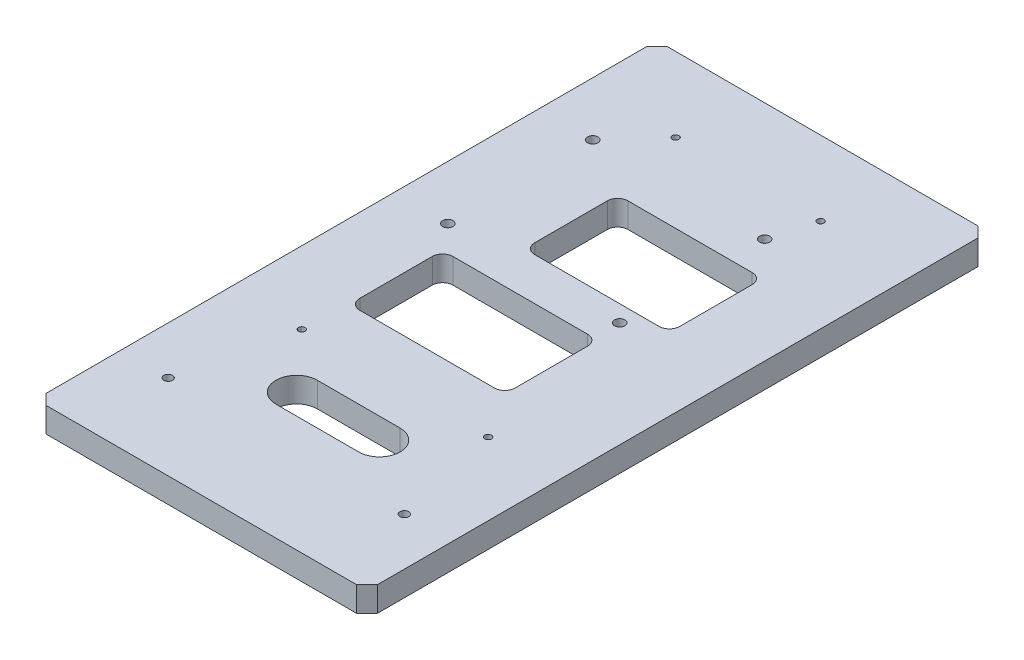
SolidWorks part; units mm, degrees
ref_plane "前视基准面" through (0, 0, 0) normal (0, 0, 1) x (1, 0, 0)
ref_plane "上视基准面" through (0, 0, 0) normal (0, 1, 0) x (1, 0, 0)
ref_plane "右视基准面" through (0, 0, 0) normal (1, 0, 0) x (0, 0, -1)
sketch "草图1" plane through (0, 0, 0) normal (0, 1, 0) x (1, 0, 0)
  line L1 (-80, 150) -> (80, 150)
  line L2 (-80, 150) -> (-80, -150)
  line L3 (-80, -150) -> (80, -150)
  line L4 (80, 150) -> (80, -150)
  line L5 (-80, 150) -> (80, -150) construction
  line L6 (-80, -150) -> (80, 150) construction
  point P0 (0, 0)
  dimension "D1" = 160
  dimension "D2" = 300
extrude "凸台-拉伸1" add sketch "草图1" along normal blind 12
sketch "草图6" plane through (0, 12, 0) normal (0, 1, 0) x (1, 0, 0)
  line L0 (-20, -84) -> (20, -84) construction
  line L1 (-20, -74) -> (20, -74)
  line L2 (-20, -94) -> (20, -94)
  line L3 (-80, 150) -> (-80, -150) construction
  line L5 (80, 150) -> (-80, 150) construction
  arc A0 (-20, -74) -> (-20, -94) centre (-20, -84) ccw
  arc A1 (20, -94) -> (20, -74) centre (20, -84) ccw
  point P2 (0, -84)
  dimension "D1" = 234
  dimension "D2" = 20
  dimension "D3" = 40
  dimension "D4" = 80
extrude "切除-拉伸1" cut sketch "草图6" against normal through all
hole_wizard "打孔尺寸(%根据)开槽圆柱头螺钉的类型3" positions "草图12" profile "草图11" counterbore size "M3" standard "GB" end condition through all
sketch "草图12" plane through (0, 0, 0) normal (0, -1, 0) x (-1, 0, 0)
  line L0 (45, -56.5) -> (-45, -56.5) construction
  line L2 (35, 114) -> (-35, 114) construction
  line L5 (0, -56.5) -> (0, 114) construction
  line L8 (-80, 150) -> (80, 150) construction
  line L10 (80, 150) -> (80, -150) construction
  point P0 (35, 114)
  point P2 (-35, 114)
  point P4 (45, -56.5)
  point P6 (-45, -56.5)
  dimension "D1" = 90
  dimension "D2" = 70
  dimension "D3" = 36
  dimension "D4" = 170.5
  dimension "D5" = 45
sketch "草图11" plane through (-35, 0, -114) normal (1, 0, 0) x (0, 0, -1)
  line L0 (0, 0) -> (0, 12)
  line L1 (0, 12) -> (1.6, 12)
  line L3 (1.6, 12) -> (1.6, 7)
  line L4 (1.6, 7) -> (3, 7)
  line L5 (3, 7) -> (3, 0)
  line L7 (3, 0) -> (0, 0)
  line L11 (0, -6.35) -> (0, 107.95) construction
  dimension "通孔孔直径" = 3.2
  dimension "通孔孔深度" = 12
  dimension "柱形沉头孔直径" = 6
  dimension "柱形沉头孔深度" = 7
sketch "草图13" plane through (0, 12, 0) normal (0, 1, 0) x (1, 0, 0)
  line L1 (54.9, 311.9539) -> (65.1, 311.9539)
  line L2 (54.9, 311.9539) -> (54.9, -278.9235)
  line L3 (54.9, -278.9235) -> (65.1, -278.9235)
  line L4 (65.1, 311.9539) -> (65.1, -278.9235)
  line L5 (54.9, 311.9539) -> (65.1, -278.9235) construction
  line L6 (54.9, -278.9235) -> (65.1, 311.9539) construction
  line L7 (-80, 150) -> (-80, -150) construction
  point P0 (60, 16.5152)
  dimension "D1" = 140
  dimension "D2" = 10.2
extrude "切除-拉伸2" [suppressed] cut sketch "草图13" against normal blind 1
hole_wizard "打孔尺寸(%根据)开槽圆柱头螺钉的类型3" positions "草图15" profile "草图14" counterbore size "M4" standard "GB"
sketch "草图15" plane through (0, 0, 0) normal (0, -1, 0) x (-1, 0, 0)
  line L1 (116, 157.5) -> (116, -157.5) construction
  point P0 (-24, -130)
  point P2 (-24, 0)
  point P4 (-24, 130)
  dimension "D1" = 130
  dimension "D2" = 140
  dimension "D3" = 130
sketch "草图14" plane through (24, 0, 130) normal (1, 0, 0) x (0, 0, -1)
  line L0 (0, 0) -> (0, 10)
  line L1 (0, 10) -> (2.25, 10)
  line L3 (2.25, 10) -> (2.25, 5)
  line L4 (2.25, 5) -> (4, 5)
  line L5 (4, 5) -> (4, 0)
  line L7 (4, 0) -> (0, 0)
  line L11 (0, -6.35) -> (0, 107.95) construction
  dimension "通孔孔直径" = 4.5
  dimension "通孔孔深度" = 10
  dimension "柱形沉头孔直径" = 8
  dimension "柱形沉头孔深度" = 5
hole_wizard "M3 螺纹孔1" positions "草图17" profile "草图16" tap size "M3" standard "GB"
sketch "草图17" plane through (0, 10, 0) normal (0, 1, 0) x (1, 0, 0)
  line L1 (17.9, 157.5) -> (-115, 157.5) construction
  line L2 (-115, 157.5) -> (-115, -157.5) construction
  point P0 (55, 87.5)
  point P2 (55, 37.5)
  dimension "D1" = 50
  dimension "D2" = 170
  dimension "D3" = 70
sketch "草图16" plane through (55, 10, -87.5) normal (1, 0, 0) x (0, 0, 1)
  line L0 (0, 0) -> (0, 10)
  line L1 (0, 10) -> (1.25, 10)
  line L2 (1.25, 10) -> (1.25, 0)
  line L5 (1.25, 0) -> (0, 0)
  line L11 (0, -6.35) -> (0, 107.95) construction
  dimension "通孔螺纹孔钻头直径" = 2.5
  dimension "通孔螺纹孔钻头深度" = 10
cosmetic thread "孔螺蚊线1" [suppressed] parameters "D2"=3
cosmetic thread "孔螺蚊线2" [suppressed] parameters "D2"=3
hole_wizard "M5 螺纹孔1" positions "草图19" profile "草图18" tap size "M5" standard "GB" end condition through all
sketch "草图19" plane through (0, 12, 0) normal (0, 1, 0) x (1, 0, 0)
  line L1 (80, 150) -> (-80, 150) construction
  line L2 (-80, 150) -> (-80, -150) construction
  point P0 (-57, -109)
  point P2 (57, -109)
  dimension "D1" = 23
  dimension "D2" = 114
  dimension "D3" = 259
sketch "草图18" plane through (-57, 12, 109) normal (1, 0, 0) x (0, 0, 1)
  line L0 (0, 0) -> (0, 12)
  line L1 (0, 12) -> (2.1, 12)
  line L2 (2.1, 12) -> (2.1, 0)
  line L5 (2.1, 0) -> (0, 0)
  line L11 (0, -6.35) -> (0, 107.95) construction
  dimension "通孔螺纹孔钻头直径" = 4.2
  dimension "通孔螺纹孔钻头深度" = 12
cosmetic thread "孔螺蚊线3" parameters "D2"=5
cosmetic thread "孔螺蚊线4" parameters "D2"=5
hole_wizard "M4 螺纹孔1" positions "草图21" profile "草图20" tap size "M4" standard "GB"
sketch "草图21" plane through (0, 0, 157.5) normal (0, 0, 1) x (1, 0, 0)
  line L1 (-116, 10) -> (116, 10) construction
  line L2 (116, 10) -> (116, 0) construction
  point P2 (34, 5)
  dimension "D1" = 82
  dimension "D2" = 5
sketch "草图20" plane through (34, 5, 157.5) normal (1, 0, 0) x (0, -1, 0)
  line L0 (0, 0) -> (0, 16.4914)
  line L1 (0, 16.4914) -> (1.65, 15.5)
  line L2 (1.65, 15.5) -> (1.65, 0)
  line L5 (1.65, 0) -> (0, 0)
  line L10 (0, 16.4914) -> (-1.65, 15.5) construction
  line L11 (0, -6.35) -> (0, 107.95) construction
  dimension "螺纹孔钻头直径" = 3.3
  dimension "螺纹孔钻头深度" = 15.5
  dimension "导头角度" = 118
cosmetic thread "孔螺蚊线5" [suppressed] parameters "D1"=12, "D2"=4
hole_wizard "M4 螺纹孔2" positions "草图23" profile "草图22" tap size "M4" standard "GB"
sketch "草图23" plane through (116, 0, 0) normal (-1, 0, 0) x (0, 0, 1)
  line L0 (-147.5, 5) -> (147.5, 5) construction
  line L3 (0, 5) -> (0, 0) construction
  point P0 (-147.5, 5)
  point P2 (147.5, 5)
  dimension "D1" = 295
  dimension "D2" = 5
sketch "草图22" plane through (116, 5, -147.5) normal (0, 1, 0) x (0, 0, -1)
  line L0 (0, 0) -> (0, 16.4914)
  line L1 (0, 16.4914) -> (1.65, 15.5)
  line L2 (1.65, 15.5) -> (1.65, 0)
  line L5 (1.65, 0) -> (0, 0)
  line L10 (0, 16.4914) -> (-1.65, 15.5) construction
  line L11 (0, -6.35) -> (0, 107.95) construction
  dimension "螺纹孔钻头直径" = 3.3
  dimension "螺纹孔钻头深度" = 15.5
  dimension "导头角度" = 118
cosmetic thread "孔螺蚊线6" [suppressed] parameters "D1"=12, "D2"=4
cosmetic thread "孔螺蚊线7" [suppressed] parameters "D1"=12, "D2"=4
hole_wizard "M4 螺纹孔3" positions "草图25" profile "草图24" tap size "M4" standard "GB"
sketch "草图25" plane through (0, 0, -157.5) normal (0, 0, -1) x (-1, 0, 0)
  line L1 (-116, 10) -> (116, 10) construction
  line L2 (-116, 10) -> (-116, 0) construction
  point P0 (-106, 5)
  point P2 (-41, 5)
  dimension "D1" = 10
  dimension "D2" = 65
  dimension "D3" = 5
sketch "草图24" plane through (106, 5, -157.5) normal (1, 0, 0) x (0, 1, 0)
  line L0 (0, 0) -> (0, 16.4914)
  line L1 (0, 16.4914) -> (1.65, 15.5)
  line L2 (1.65, 15.5) -> (1.65, 0)
  line L5 (1.65, 0) -> (0, 0)
  line L10 (0, 16.4914) -> (-1.65, 15.5) construction
  line L11 (0, -6.35) -> (0, 107.95) construction
  dimension "螺纹孔钻头直径" = 3.3
  dimension "螺纹孔钻头深度" = 15.5
  dimension "导头角度" = 118
cosmetic thread "孔螺蚊线8" [suppressed] parameters "D1"=12, "D2"=4
cosmetic thread "孔螺蚊线14" [suppressed] parameters "D1"=12, "D2"=4
chamfer "倒角1" distance 5 angle 45 4 edges at (-80, 6, -150) (80, 6, -150) (-80, 6, 150) (80, 6, 150)
hole_wizard "M8 螺纹孔1" positions "草图28" profile "草图27" tap size "M8" standard "GB"
sketch "草图28" plane through (0, 10, 0) normal (0, 1, 0) x (1, 0, 0)
  line L0 (-96, 132.5) -> (96, 132.5) construction
  line L1 (96, 132.5) -> (96, -132.5) construction
  line L4 (0, 0) -> (0, 132.5) construction
  line L7 (0, 0) -> (96, 0) construction
  line L10 (-116, 152.5) -> (-116, -152.5) construction
  line L11 (111, 157.5) -> (-111, 157.5) construction
  point P0 (-96, 132.5)
  point P2 (96, 132.5)
  point P4 (-96, -132.5)
  point P6 (96, -132.5)
  dimension "D1" = 20
  dimension "D2" = 25
sketch "草图27" plane through (-96, 10, -132.5) normal (1, 0, 0) x (0, 0, 1)
  line L0 (0, 0) -> (0, 10)
  line L1 (0, 10) -> (3.4, 10)
  line L2 (3.4, 10) -> (3.4, 0)
  line L5 (3.4, 0) -> (0, 0)
  line L11 (0, -6.35) -> (0, 107.95) construction
  dimension "通孔螺纹孔钻头直径" = 6.8
  dimension "通孔螺纹孔钻头深度" = 10
cosmetic thread "孔螺蚊线10" [suppressed] parameters "D2"=8
cosmetic thread "孔螺蚊线11" [suppressed] parameters "D2"=8
cosmetic thread "孔螺蚊线12" [suppressed] parameters "D2"=8
cosmetic thread "孔螺蚊线13" [suppressed] parameters "D2"=8
sketch "草图29" plane through (0, 12, 0) normal (0, 1, 0) x (1, 0, 0)
  line L0 (-80, 145) -> (-80, -145) construction
  line L1 (-25, 76) -> (45, 76)
  line L2 (-25, 76) -> (-25, 31)
  line L3 (-25, 31) -> (45, 31)
  line L4 (45, 76) -> (45, 31)
  line L5 (-25, 76) -> (45, 31) construction
  line L6 (-25, 31) -> (45, 76) construction
  line L7 (-44, 10.5) -> (31, 10.5)
  line L8 (-44, 10.5) -> (-44, -34.5)
  line L9 (-44, -34.5) -> (31, -34.5)
  line L10 (31, 10.5) -> (31, -34.5)
  line L11 (-44, 10.5) -> (31, -34.5) construction
  line L12 (-44, -34.5) -> (31, 10.5) construction
  line L13 (75, 150) -> (-75, 150) construction
  point P0 (10, 53.5)
  point P5 (-6.5, -12)
  dimension "D1" = 55
  dimension "D2" = 45
  dimension "D3" = 70
  dimension "D4" = 74
  dimension "D5" = 139.5
  dimension "D6" = 75
  dimension "D7" = 45
  dimension "D8" = 36
extrude "切除-拉伸3" cut sketch "草图29" against normal through all
fillet "圆角1" radius 5 8 edges at (45, 6, -76) (45, 6, -31) (-25, 6, -76) (-44, 6, -10.5) (31, 6, -10.5) (31, 6, 34.5) (-44, 6, 34.5) (-25, 6, -31)
hole_wizard "M4 螺纹孔4" positions "草图31" profile "草图30" tap size "M4" standard "GB"
sketch "草图31" plane through (0, 10, 0) normal (0, 1, 0) x (1, 0, 0)
  line L0 (28.1, -157.5) -> (110, -157.5) construction
  line L1 (115, -152.5) -> (115, 152.5) construction
  point P0 (80, -16.5)
  dimension "D1" = 141
  dimension "D2" = 35
sketch "草图30" plane through (80, 10, 16.5) normal (1, 0, 0) x (0, 0, 1)
  line L0 (0, 0) -> (0, 10)
  line L1 (0, 10) -> (1.65, 10)
  line L2 (1.65, 10) -> (1.65, 0)
  line L5 (1.65, 0) -> (0, 0)
  line L11 (0, -6.35) -> (0, 107.95) construction
  dimension "通孔螺纹孔钻头直径" = 3.3
  dimension "通孔螺纹孔钻头深度" = 10
cosmetic thread "孔螺蚊线15" [suppressed] parameters "D2"=4
hole_wizard "M4 螺纹孔5" positions "草图33" profile "草图32" tap size "M4" standard "GB"
sketch "草图33" plane through (0, 10, 0) normal (0, 1, 0) x (1, 0, 0)
  line L0 (100, -54) -> (100, -29) construction
  line L3 (100, -41.5) -> (110.4761, -41.5) construction
  line L6 (116, -152.5) -> (116, 152.5) construction
  line L7 (-111, -157.5) -> (111, -157.5) construction
  point P0 (100, -54)
  point P2 (100, -29)
  dimension "D1" = 16
  dimension "D2" = 116
  dimension "D3" = 25
sketch "草图32" plane through (100, 10, 54) normal (1, 0, 0) x (0, 0, 1)
  line L0 (0, 0) -> (0, 10)
  line L1 (0, 10) -> (1.65, 10)
  line L2 (1.65, 10) -> (1.65, 0)
  line L5 (1.65, 0) -> (0, 0)
  line L11 (0, -6.35) -> (0, 107.95) construction
  dimension "通孔螺纹孔钻头直径" = 3.3
  dimension "通孔螺纹孔钻头深度" = 10
cosmetic thread "孔螺蚊线16" [suppressed] parameters "D2"=4
cosmetic thread "孔螺蚊线17" [suppressed] parameters "D2"=4
sketch "草图34" [suppressed] plane through (0, 10, 0) normal (0, 1, 0) x (1, 0, 0)
  line L0 (24, 162.5) -> (24, 152.5) construction
  line L1 (29.1, 157.5) -> (18.9, 157.5) construction
  line L2 (28, 162.5) -> (28, 152.5)
  line L3 (20, 162.5) -> (20, 152.5)
  line L4 (111, 157.5) -> (29.1, 157.5) construction
  arc A0 (28, 162.5) -> (20, 162.5) centre (24, 162.5) ccw
  arc A1 (20, 152.5) -> (28, 152.5) centre (24, 152.5) ccw
  point P4 (24, 157.5)
  dimension "D1" = 8
  dimension "D2" = 5
extrude "切除-拉伸4" [suppressed] cut sketch "草图34" against normal through all
sketch "草图35" plane through (0, 12, 0) normal (0, 1, 0) x (1, 0, 0)
  line L0 (15, 5) -> (55, 5) construction
  line L1 (15, 15) -> (55, 15)
  line L2 (15, -5) -> (55, -5)
  line L3 (80, -145) -> (80, 145) construction
  line L4 (-75, -150) -> (75, -150) construction
  arc A0 (15, 15) -> (15, -5) centre (15, 5) ccw
  arc A1 (55, -5) -> (55, 15) centre (55, 5) ccw
  point P2 (35, 5)
  dimension "D1" = 20
  dimension "D2" = 40
  dimension "D3" = 25
  dimension "D4" = 155
extrude "切除-拉伸5" [suppressed] cut sketch "草图35" against normal through all
sketch "草图36" plane through (0, 0, 150) normal (0, 0, 1) x (1, 0, 0)
  line L0 (-75, 12) -> (75, 12) construction
  line L1 (-80, 0) -> (-80, 12) construction
  circle A0 centre (-65, 7) radius 4
  dimension "D1" = 8
  dimension "D2" = 5
  dimension "D3" = 15
extrude "切除-拉伸6" [suppressed] cut sketch "草图36" against normal blind 4
mirror "镜向1" [suppressed] about plane through (0, 0, 0) normal (0, 0, 1)
hole_wizard "M6 螺纹孔1" positions "草图38" profile "草图37" tap size "M6" standard "GB" end condition through all
sketch "草图38" plane through (0, 12, 0) normal (0, 1, 0) x (1, 0, 0)
  line L6 (-80, 145) -> (-80, -145) construction
  line L7 (75, 150) -> (-75, 150) construction
  point P0 (-54, 93)
  point P2 (29, 93)
  point P4 (-54, 23)
  point P6 (29, 23)
  dimension "D1" = 83
  dimension "D2" = 70
  dimension "D3" = 26
  dimension "D4" = 57
sketch "草图37" plane through (-54, 12, -93) normal (1, 0, 0) x (0, 0, 1)
  line L0 (0, 0) -> (0, 12)
  line L1 (0, 12) -> (2.5, 12)
  line L2 (2.5, 12) -> (2.5, 0)
  line L5 (2.5, 0) -> (0, 0)
  line L11 (0, -6.35) -> (0, 107.95) construction
  dimension "通孔螺纹孔钻头直径" = 5
  dimension "通孔螺纹孔钻头深度" = 12
cosmetic thread "孔螺蚊线18" parameters "D2"=6
cosmetic thread "孔螺蚊线19" parameters "D2"=6
cosmetic thread "孔螺蚊线20" parameters "D2"=6
cosmetic thread "孔螺蚊线21" parameters "D2"=6
hole_wizard "M4 螺纹孔6" positions "草图40" profile "草图39" tap size "M4" standard "GB"
sketch "草图40" plane through (0, 12, 0) normal (0, 1, 0) x (1, 0, 0)
  point P0 (-70.5, 98)
  point P3 (70.5, 98)
  point P6 (70.5, -63)
  point P9 (-70.5, -63)
sketch "草图39" plane through (-70.5, 12, -98) normal (1, 0, 0) x (0, 0, 1)
  line L0 (0, 0) -> (0, 12)
  line L1 (0, 12) -> (1.65, 12)
  line L2 (1.65, 12) -> (1.65, 0)
  line L5 (1.65, 0) -> (0, 0)
  line L11 (0, -6.35) -> (0, 107.95) construction
  dimension "通孔螺纹孔钻头直径" = 3.3
  dimension "通孔螺纹孔钻头深度" = 12
cosmetic thread "孔螺蚊线22" [suppressed] parameters "D2"=4
cosmetic thread "孔螺蚊线23" [suppressed] parameters "D2"=4
cosmetic thread "孔螺蚊线24" [suppressed] parameters "D2"=4
cosmetic thread "孔螺蚊线25" [suppressed] parameters "D2"=4
